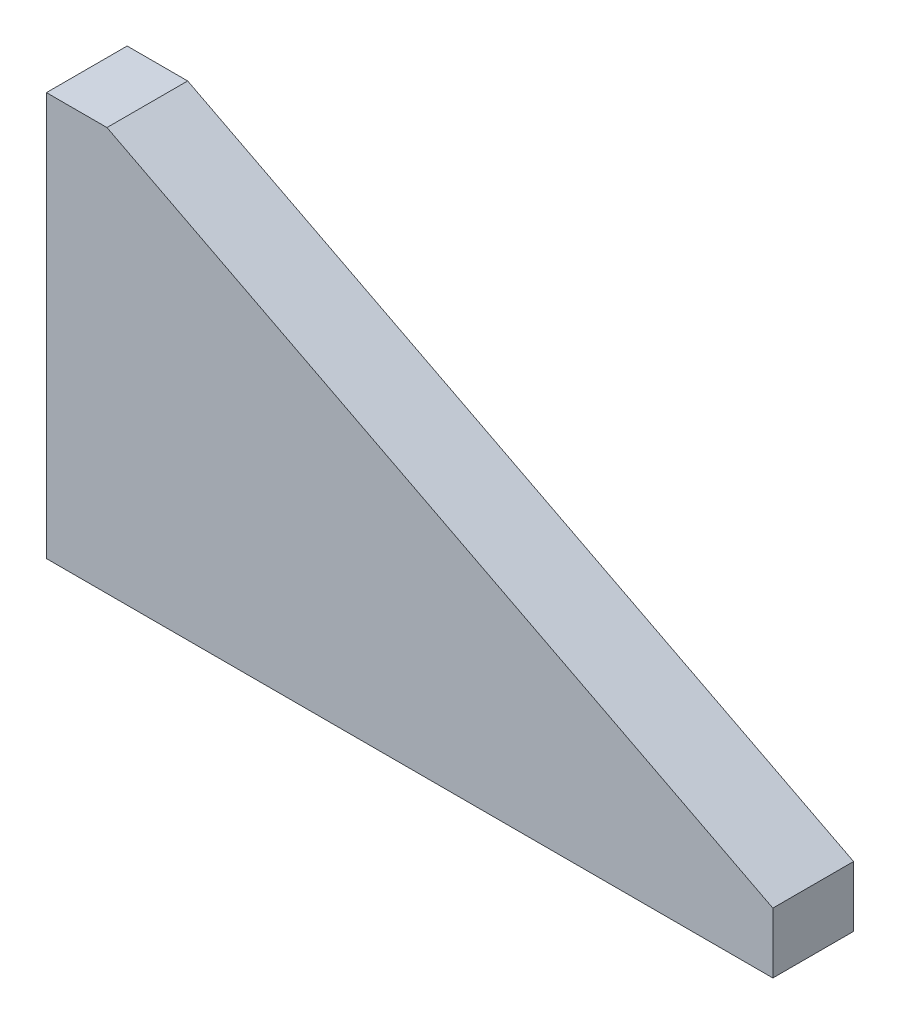
from build123d import *

# Parameters (mm, degrees)
BOSS_EXTRUDE1_DEPTH = 20


with BuildPart() as part:
    # Sketch1 → Boss-Extrude1 (new body)
    with BuildSketch(Plane.XY):
        Polygon((0, 0), (0, 100), (15, 100), (180, 15), (180, 0), align=None)
    extrude(amount=BOSS_EXTRUDE1_DEPTH)


solid = part.part
